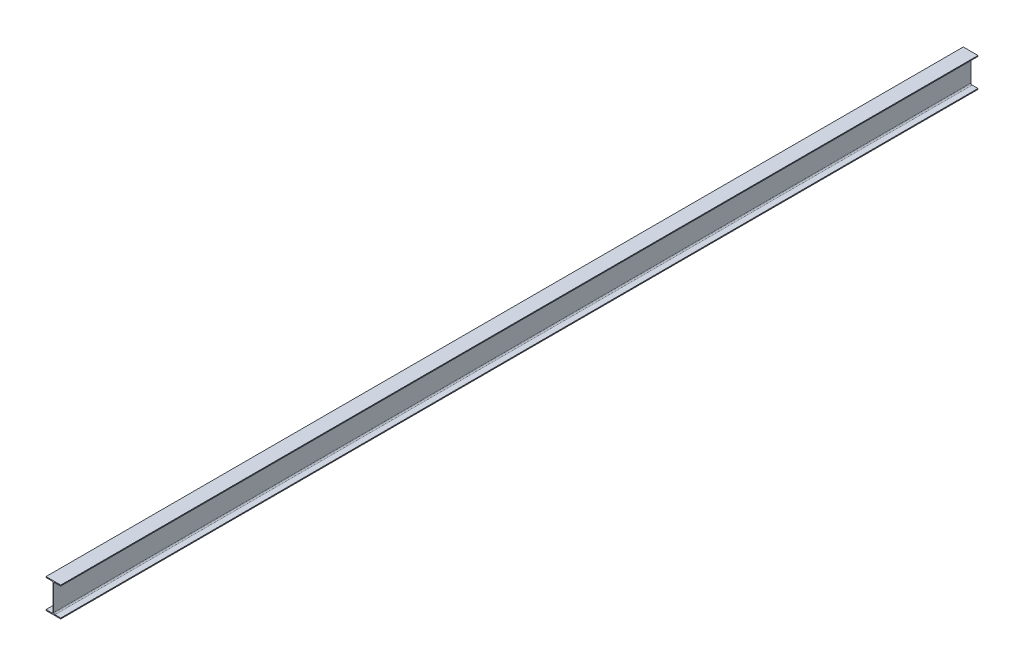
SolidWorks part; units mm, degrees
ref_plane "Front Plane" through (0, 0, 0) normal (0, 0, 1) x (1, 0, 0)
ref_plane "Top Plane" through (0, 0, 0) normal (0, 1, 0) x (1, 0, 0)
ref_plane "Right Plane" through (0, 0, 0) normal (1, 0, 0) x (0, 0, -1)
other "Configuration Table"
sketch "Sketch1" plane through (0, 0, 0) normal (0, 0, 1) x (1, 0, 0)
  line L0 (0, 0) -> (0, 300) construction
  line L1 (75, 0) -> (-75, 0)
  line L2 (-75, 0) -> (-75, 9)
  line L3 (-75, 9) -> (-16.25, 9)
  line L4 (3.25, 22) -> (3.25, 278)
  line L6 (-75, 291) -> (-75, 300)
  line L7 (-75, 300) -> (75, 300)
  line L8 (-3.25, 22) -> (-3.25, 278)
  line L9 (75, 291) -> (75, 300)
  line L10 (16.25, 291) -> (75, 291)
  line L11 (75, 9) -> (16.25, 9)
  line L12 (75, 0) -> (75, 9)
  line L13 (-16.25, 291) -> (-75, 291)
  arc A0 (16.25, 9) -> (3.25, 22) centre (16.25, 22) cw
  arc A1 (-3.25, 22) -> (-16.25, 9) centre (-16.25, 22) cw
  arc A2 (3.25, 278) -> (16.25, 291) centre (16.25, 278) cw
  arc A3 (-3.25, 278) -> (-16.25, 291) centre (-16.25, 278) ccw
  point P18 (3.25, 9)
  point P21 (-3.25, 9)
  point P24 (3.25, 291)
  point P27 (-3.25, 291)
  dimension "D6" = 13
  dimension "D1" = 300
  dimension "D2" = 150
  dimension "D3" = 6.5
  dimension "D4" = 9
  dimension "D5" = 9
extrude "Boss-Extrude1" add sketch "Sketch1" along normal blind 9347
